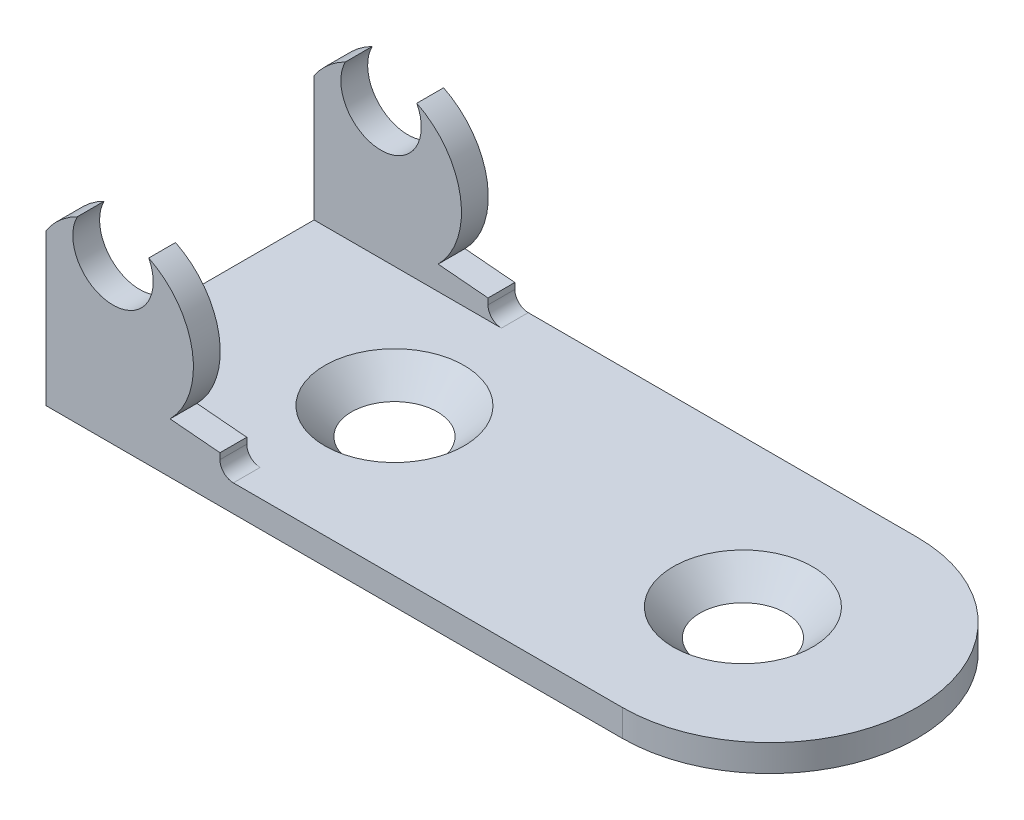
from build123d import *

# Parameters (mm, degrees)
EXTRUDE_1_DEPTH      = 5.5
EXTRUDE_1_DEPTH_BACK = 5.5
SKETCH_2_W           = 108
SKETCH_2_H           = 22
CUT_EXTRUDE_1_DEPTH  = 11
SKETCH_4_W           = 9
SKETCH_4_H           = 10
CUT_EXTRUDE_2_DEPTH  = 11


with BuildPart() as part:
    # 草图1 → 凸台-拉伸1 (new, two sides: drawn at the far end of the back side and taken through both)
    with BuildSketch(Plane.XY.offset(-EXTRUDE_1_DEPTH_BACK)):
        with BuildLine():
            Line((0, 0), (27, 0))
            Line((27, 0), (27, 1))
            Line((27, 1), (6.99, 1))
            ThreePointArc((6.99, 1), (6.636446609, 1.146446609), (6.49, 1.5))
            Line((6.49, 1.5), (6.49, 1.724666059))
            Line((6.49, 1.724666059), (4.63, 1.887394973))
            ThreePointArc((4.63, 1.887394973), (5.459499899, 4.491284383), (3.833170563, 6.6875))
            ThreePointArc((3.833170563, 6.6875), (2.5, 4.5), (1.166829437, 6.6875))
            ThreePointArc((1.166829437, 6.6875), (0.515533844, 6.249865346), (0, 5.658312395))
            Line((0, 5.658312395), (0, 0))
        make_face()
    extrude(amount=EXTRUDE_1_DEPTH + EXTRUDE_1_DEPTH_BACK)

    # 草图2 → 切除-拉伸1 (cut)
    with BuildSketch(Plane(origin=(0, 0, 0), x_dir=(1, 0, 0), z_dir=(0, 1, 0))):
        Rectangle(SKETCH_2_W, SKETCH_2_H)
        with BuildLine():
            Line((0, 5.5), (0, -5.5))
            Line((0, -5.5), (21.5, -5.5))
            ThreePointArc((21.5, -5.5), (27, 0), (21.5, 5.5))
            Line((21.5, 5.5), (0, 5.5))
        make_face(mode=Mode.SUBTRACT)
    extrude(amount=CUT_EXTRUDE_1_DEPTH, mode=Mode.SUBTRACT)

    # 草图4 → 切除-拉伸2 (cut)
    with BuildSketch(Plane(origin=(0, 0, 0), x_dir=(0, 0, -1), z_dir=(1, 0, 0))):
        with Locations((0, 6)):
            Rectangle(SKETCH_4_W, SKETCH_4_H)
    extrude(amount=CUT_EXTRUDE_2_DEPTH, mode=Mode.SUBTRACT)

    # 草图3 → 切除-旋转1 (revolve, cut)
    with BuildSketch(Plane.XY, mode=Mode.PRIVATE) as cut_revolve_1_sk:
        Polygon((7.5, 1), (10.1, 1), (9.1, 0), (7.5, 0), align=None)
    revolve(cut_revolve_1_sk.sketch.rotate(Axis((7.5, 0, 0), (0, 1, 0)), 270), axis=Axis((7.5, 0, 0), (0, 1, 0)), mode=Mode.SUBTRACT)

    # 草图5 → 切除-旋转2 (revolve, cut)
    with BuildSketch(Plane.XY, mode=Mode.PRIVATE) as cut_revolve_2_sk:
        Polygon((20.5, 1), (23.1, 1), (22.1, 0), (20.5, 0), align=None)
    revolve(cut_revolve_2_sk.sketch.rotate(Axis((20.5, 0, 0), (0, 1, 0)), 270), axis=Axis((20.5, 0, 0), (0, 1, 0)), mode=Mode.SUBTRACT)


solid = part.part
